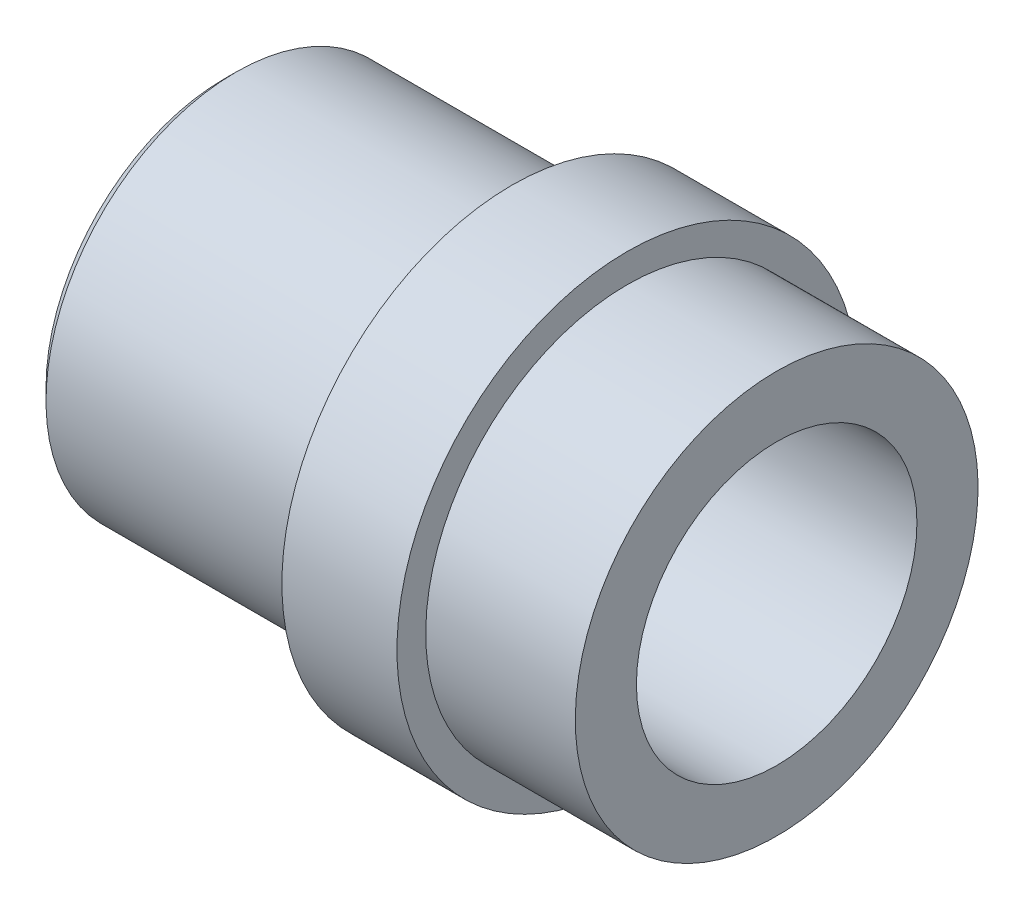
SolidWorks part; units mm, degrees
ref_plane "Front Plane" through (0, 0, 0) normal (0, 0, 1) x (1, 0, 0)
ref_plane "Top Plane" through (0, 0, 0) normal (0, 1, 0) x (1, 0, 0)
ref_plane "Right Plane" through (0, 0, 0) normal (1, 0, 0) x (0, 0, -1)
sketch "Sketch1" plane through (0, 0, 0) normal (0, 0, 1) x (1, 0, 0)
  line L0 (0, 0) -> (-25.4468, 0) construction
  line L1 (-48, 0) -> (-48, 15.5)
  line L2 (-47, 16.5) -> (-23, 16.5)
  line L3 (-23, 16.5) -> (-23, 20)
  line L4 (-23, 20) -> (-13, 20)
  line L5 (-13, 20) -> (-13, 17.5)
  line L6 (-13, 17.5) -> (0, 17.5)
  line L7 (0, 17.5) -> (0, 0)
  line L8 (-48, 15.5) -> (-47, 16.5)
  line L9 (-48, 0) -> (0, 0)
  point P4 (-48, 16.5)
  dimension "D1" = 20
  dimension "D2" = 17.5
  dimension "D3" = 16.5
  dimension "D4" = 0
  dimension "D5" = 13
  dimension "D6" = 48
  dimension "D7" = 25
  dimension "D8" = 0
revolve "Revolve1" add sketch "Sketch1" angle 360 about L0
sketch "Sketch2" plane through (0, 0, 0) normal (1, 0, 0) x (0, 0, -1)
  circle A0 centre (0, 0) radius 10.25
  dimension "D1" = 20.5
extrude "Cut-Extrude1" cut sketch "Sketch2" against normal through all
sketch "Sketch4" plane through (0, 0, 0) normal (1, 0, 0) x (0, 0, -1)
  circle A0 centre (0, 0) radius 12.1888
extrude "Cut-Extrude2" cut sketch "Sketch4" against normal blind 20
